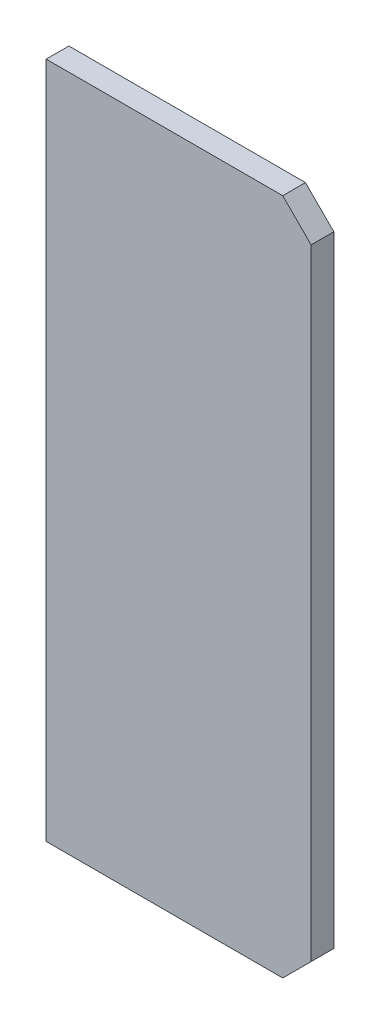
from build123d import *

# Parameters (mm, degrees)
SKETCH1_W           = 140
SKETCH1_H           = 358
BOSS_EXTRUDE1_DEPTH = 12
CHAMFER2_SIZE       = 15


with BuildPart() as part:
    # Sketch1 → Boss-Extrude1 (new body)
    with BuildSketch(Plane.XY):
        with Locations((70, 179)):
            Rectangle(SKETCH1_W, SKETCH1_H)
    extrude(amount=BOSS_EXTRUDE1_DEPTH)

    # Chamfer2
    chamfer2_edges = [part.edges().sort_by_distance(p)[0] for p in [
        (140, 358, 6),
        (140, 0, 6),
    ]]
    chamfer(chamfer2_edges, length=CHAMFER2_SIZE)


solid = part.part
